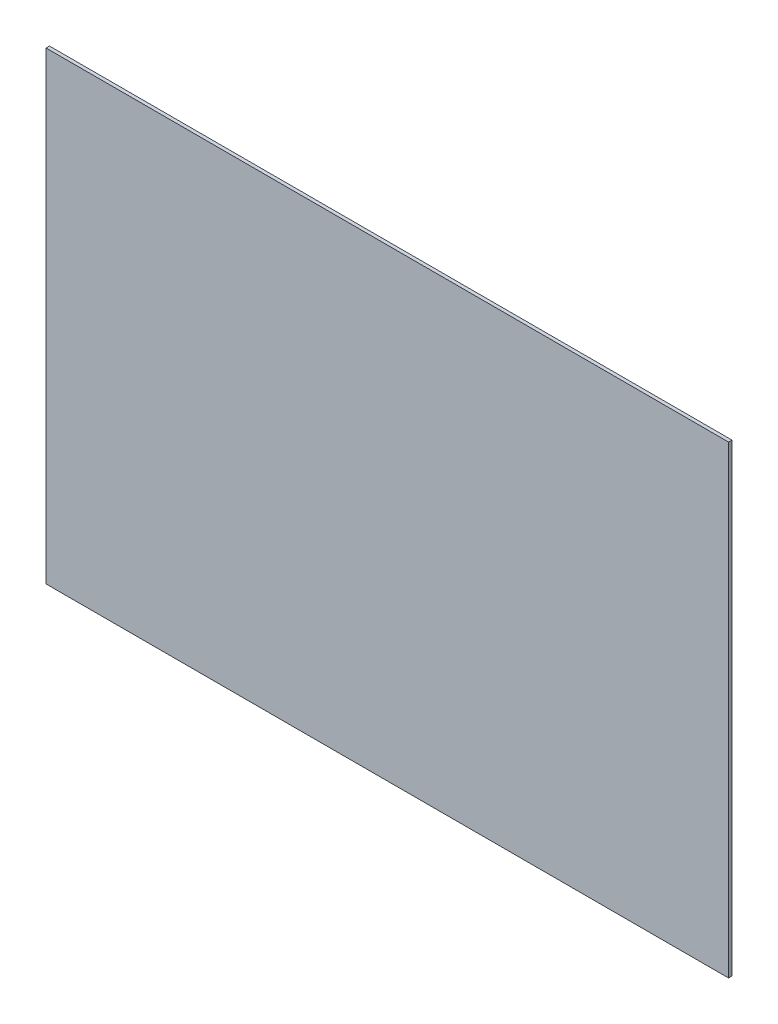
from build123d import *

# Parameters (mm, degrees)
SKETCH_1_W      = 997
SKETCH_1_H      = 678
EXTRUDE_1_DEPTH = 5


with BuildPart() as part:
    # 草图1 → 凸台-拉伸1 (new body)
    with BuildSketch(Plane.XY):
        Rectangle(SKETCH_1_W, SKETCH_1_H)
    extrude(amount=EXTRUDE_1_DEPTH)


solid = part.part
